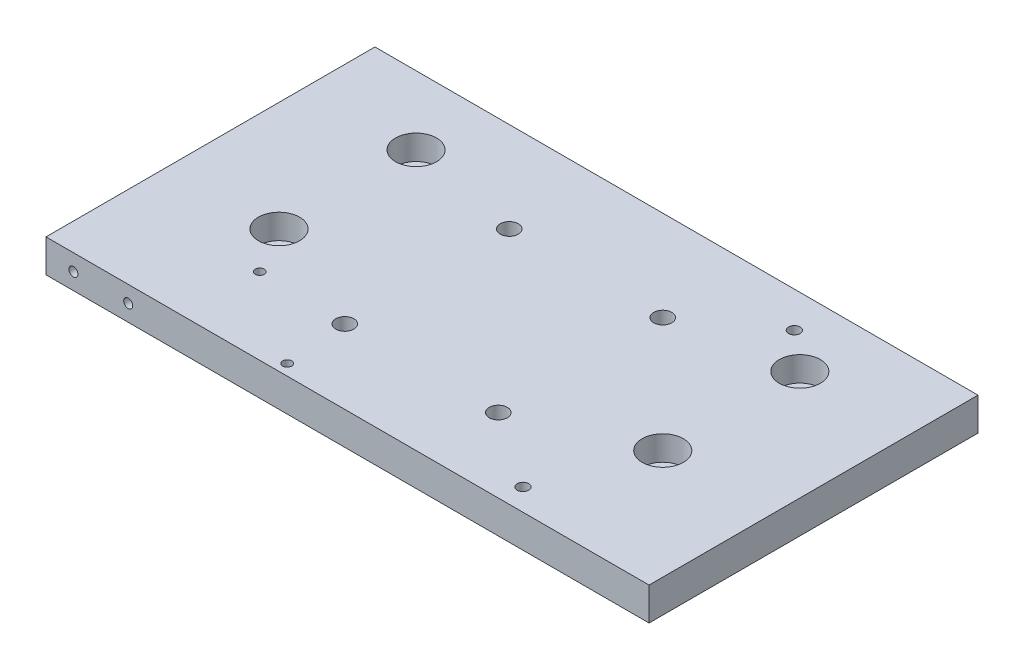
SolidWorks part; units mm, degrees
material "6061 合金"
ref_plane "前视基准面" through (0, 0, 0) normal (0, 0, 1) x (1, 0, 0)
ref_plane "上视基准面" through (0, 0, 0) normal (0, 1, 0) x (1, 0, 0)
ref_plane "右视基准面" through (0, 0, 0) normal (1, 0, 0) x (0, 0, -1)
sketch "草图1" plane through (0, 0, 0) normal (0, 0, 1) x (1, 0, 0)
  line L1 (-110, 6) -> (110, 6)
  line L2 (-110, 6) -> (-110, -6)
  line L3 (-110, -6) -> (110, -6)
  line L4 (110, 6) -> (110, -6)
  line L5 (-110, 6) -> (110, -6) construction
  line L6 (-110, -6) -> (110, 6) construction
  point P0 (0, 0)
  dimension "D1" = 220
  dimension "D2" = 12
extrude "凸台-拉伸1" add sketch "草图1" along normal mid plane 120
hole_wizard "M6 螺纹孔1" positions "3D草图1" profile "草图2" tap size "M6" standard "GB"
sketch3d "3D草图1"
  line L1 (-110, 6, -60) -> (-110, -6, -60) construction
  line L2 (110, -6, -60) -> (110, 6, -60) construction
  line L3 (-110, -6, -60) -> (110, -6, -60) construction
  point P0 (70, 0, -60)
  point P2 (0, 0, -60)
  point P4 (-70, 0, -60)
  dimension "D1" = 40
  dimension "D2" = 110
  dimension "D3" = 40
  dimension "D4" = 6
  dimension "D5" = 6
  dimension "D6" = 6
sketch "草图2" plane through (70, 0, -60) normal (1, 0, 0) x (0, 1, 0)
  line L0 (0, 0) -> (0, 14.5022)
  line L1 (0, 14.5022) -> (2.5, 13)
  line L2 (2.5, 13) -> (2.5, 0)
  line L5 (2.5, 0) -> (0, 0)
  line L10 (0, 14.5022) -> (-2.5, 13) construction
  line L11 (0, -6.35) -> (0, 107.95) construction
  dimension "螺纹孔钻头直径" = 5
  dimension "螺纹孔钻头深度" = 13
  dimension "导头角度" = 118
cosmetic thread "孔螺蚊线1" parameters "D1"=10, "D2"=8
cosmetic thread "孔螺蚊线2" parameters "D1"=10, "D2"=8
cosmetic thread "孔螺蚊线3" parameters "D1"=10, "D2"=8
hole_wizard "打孔尺寸(%根据)内六角圆柱头螺钉的类型2" positions "3D草图2" profile "草图4" counterbore size "M8" standard "GB" end condition through all
sketch3d "3D草图2"
  line L0 (-110, 6, 60) -> (-110, 6, -60) construction
  line L1 (110, 6, -60) -> (-110, 6, -60) construction
  line L2 (110, 6, 60) -> (-110, 6, 60) construction
  line L3 (110, 6, 60) -> (110, 6, -60) construction
  point P0 (-70, 6, -35)
  point P2 (-70, 6, 15)
  point P4 (70, 6, -35)
  point P6 (70, 6, 15)
  dimension "D1" = 40
  dimension "D2" = 40
  dimension "D3" = 25
  dimension "D4" = 45
  dimension "D5" = 40
  dimension "D6" = 25
  dimension "D7" = 40
  dimension "D8" = 45
sketch "草图4" plane through (-70, 6, -35) normal (1, 0, 0) x (0, 0, 1)
  line L0 (0, 0) -> (0, 12)
  line L1 (0, 12) -> (4.5, 12)
  line L3 (4.5, 12) -> (4.5, 9)
  line L4 (4.5, 9) -> (7.5, 9)
  line L5 (7.5, 9) -> (7.5, 0)
  line L7 (7.5, 0) -> (0, 0)
  line L11 (0, -6.35) -> (0, 107.95) construction
  dimension "通孔孔直径" = 9
  dimension "通孔孔深度" = 12
  dimension "柱形沉头孔直径" = 15
  dimension "柱形沉头孔深度" = 9
sketch "草图5" plane through (0, -6, 0) normal (0, -1, 0) x (1, 0, 0)
  line L1 (-28, 33) -> (28, 33)
  line L2 (-28, 33) -> (-28, -27)
  line L3 (-28, -27) -> (28, -27)
  line L4 (28, 33) -> (28, -27)
  line L5 (-28, 33) -> (28, -27) construction
  line L6 (-28, -27) -> (28, 33) construction
  point P0 (0, 3)
  dimension "D1" = 56
  dimension "D2" = 60
  dimension "D3" = 3
hole_wizard "打孔尺寸(%根据)内六角圆柱头螺钉的类型2" positions "3D草图3" profile "草图6" counterbore size "M6" standard "GB" end condition through all
sketch3d "3D草图3"
  point P2 (-28, -6, -27)
  point P5 (28, -6, -27)
  point P8 (28, -6, 33)
  point P13 (-28, -6, 33)
sketch "草图6" plane through (-28, -6, -27) normal (1, 0, 0) x (0, 0, -1)
  line L0 (0, 0) -> (0, 12)
  line L1 (0, 12) -> (3.3, 12)
  line L3 (3.3, 12) -> (3.3, 6.8)
  line L4 (3.3, 6.8) -> (5.5, 6.8)
  line L5 (5.5, 6.8) -> (5.5, 0)
  line L7 (5.5, 0) -> (0, 0)
  line L11 (0, -6.35) -> (0, 107.95) construction
  dimension "通孔孔直径" = 6.6
  dimension "通孔孔深度" = 12
  dimension "柱形沉头孔直径" = 11
  dimension "柱形沉头孔深度" = 6.8
hole_wizard "M4 螺纹孔1" positions "草图8" profile "草图7" tap size "M4" standard "GB" end condition through all
sketch "草图8" plane through (0, -6, 0) normal (0, -1, 0) x (-1, 0, 0)
  line L0 (110, -60) -> (-110, -60) construction
  line L1 (110, -60) -> (110, 60) construction
  point P0 (26, -56)
  point P2 (60, -32)
  dimension "D1" = 4
  dimension "D2" = 84
  dimension "D3" = 50
  dimension "D4" = 24
sketch "草图7" plane through (-26, -6, 56) normal (1, 0, 0) x (0, 0, -1)
  line L0 (0, 0) -> (0, 12)
  line L1 (0, 12) -> (1.65, 12)
  line L2 (1.65, 12) -> (1.65, 0)
  line L5 (1.65, 0) -> (0, 0)
  line L11 (0, -6.35) -> (0, 107.95) construction
  dimension "通孔螺纹孔钻头直径" = 3.3
  dimension "通孔螺纹孔钻头深度" = 12
cosmetic thread "孔螺蚊线6" parameters "D2"=4
cosmetic thread "孔螺蚊线7" parameters "D2"=4
hole_wizard "M5 螺纹孔2" positions "草图10" profile "草图11" tap size "M5" standard "GB" end condition through all
sketch "草图10" plane through (0, -6, 0) normal (0, -1, 0) x (-1, 0, 0)
  line L0 (-110, -60) -> (-110, 60) construction
  line L1 (110, -60) -> (-110, -60) construction
  point P0 (-56, -52)
  point P2 (-56, 47)
  dimension "D1" = 54
  dimension "D2" = 8
  dimension "D3" = 99
sketch "草图11" plane through (56, -6, 52) normal (1, 0, 0) x (0, 0, -1)
  line L0 (0, 0) -> (0, 12)
  line L1 (0, 12) -> (2.1, 12)
  line L2 (2.1, 12) -> (2.1, 0)
  line L5 (2.1, 0) -> (0, 0)
  line L11 (0, -6.35) -> (0, 107.95) construction
  dimension "通孔螺纹孔钻头直径" = 4.2
  dimension "通孔螺纹孔钻头深度" = 12
cosmetic thread "孔螺蚊线4" parameters "D2"=5
cosmetic thread "孔螺蚊线5" parameters "D2"=5
hole_wizard "M4 螺纹孔2" positions "草图13" profile "草图12" tap size "M4" standard "GB"
sketch "草图13" plane through (0, 0, 60) normal (0, 0, 1) x (1, 0, 0)
  line L0 (-110, 6) -> (-110, -6) construction
  point P0 (-100, 0)
  point P2 (-80, 0)
  dimension "D1" = 20
  dimension "D2" = 10
sketch "草图12" plane through (-100, 0, 60) normal (1, 0, 0) x (0, -1, 0)
  line L0 (0, 0) -> (0, 11.0914)
  line L1 (0, 11.0914) -> (1.65, 10.1)
  line L2 (1.65, 10.1) -> (1.65, 0)
  line L5 (1.65, 0) -> (0, 0)
  line L10 (0, 11.0914) -> (-1.65, 10.1) construction
  line L11 (0, -6.35) -> (0, 107.95) construction
  dimension "螺纹孔钻头直径" = 3.3
  dimension "螺纹孔钻头深度" = 10.1
  dimension "导头角度" = 118
cosmetic thread "孔螺蚊线8" parameters "D1"=8, "D2"=4
cosmetic thread "孔螺蚊线9" parameters "D1"=8, "D2"=4
